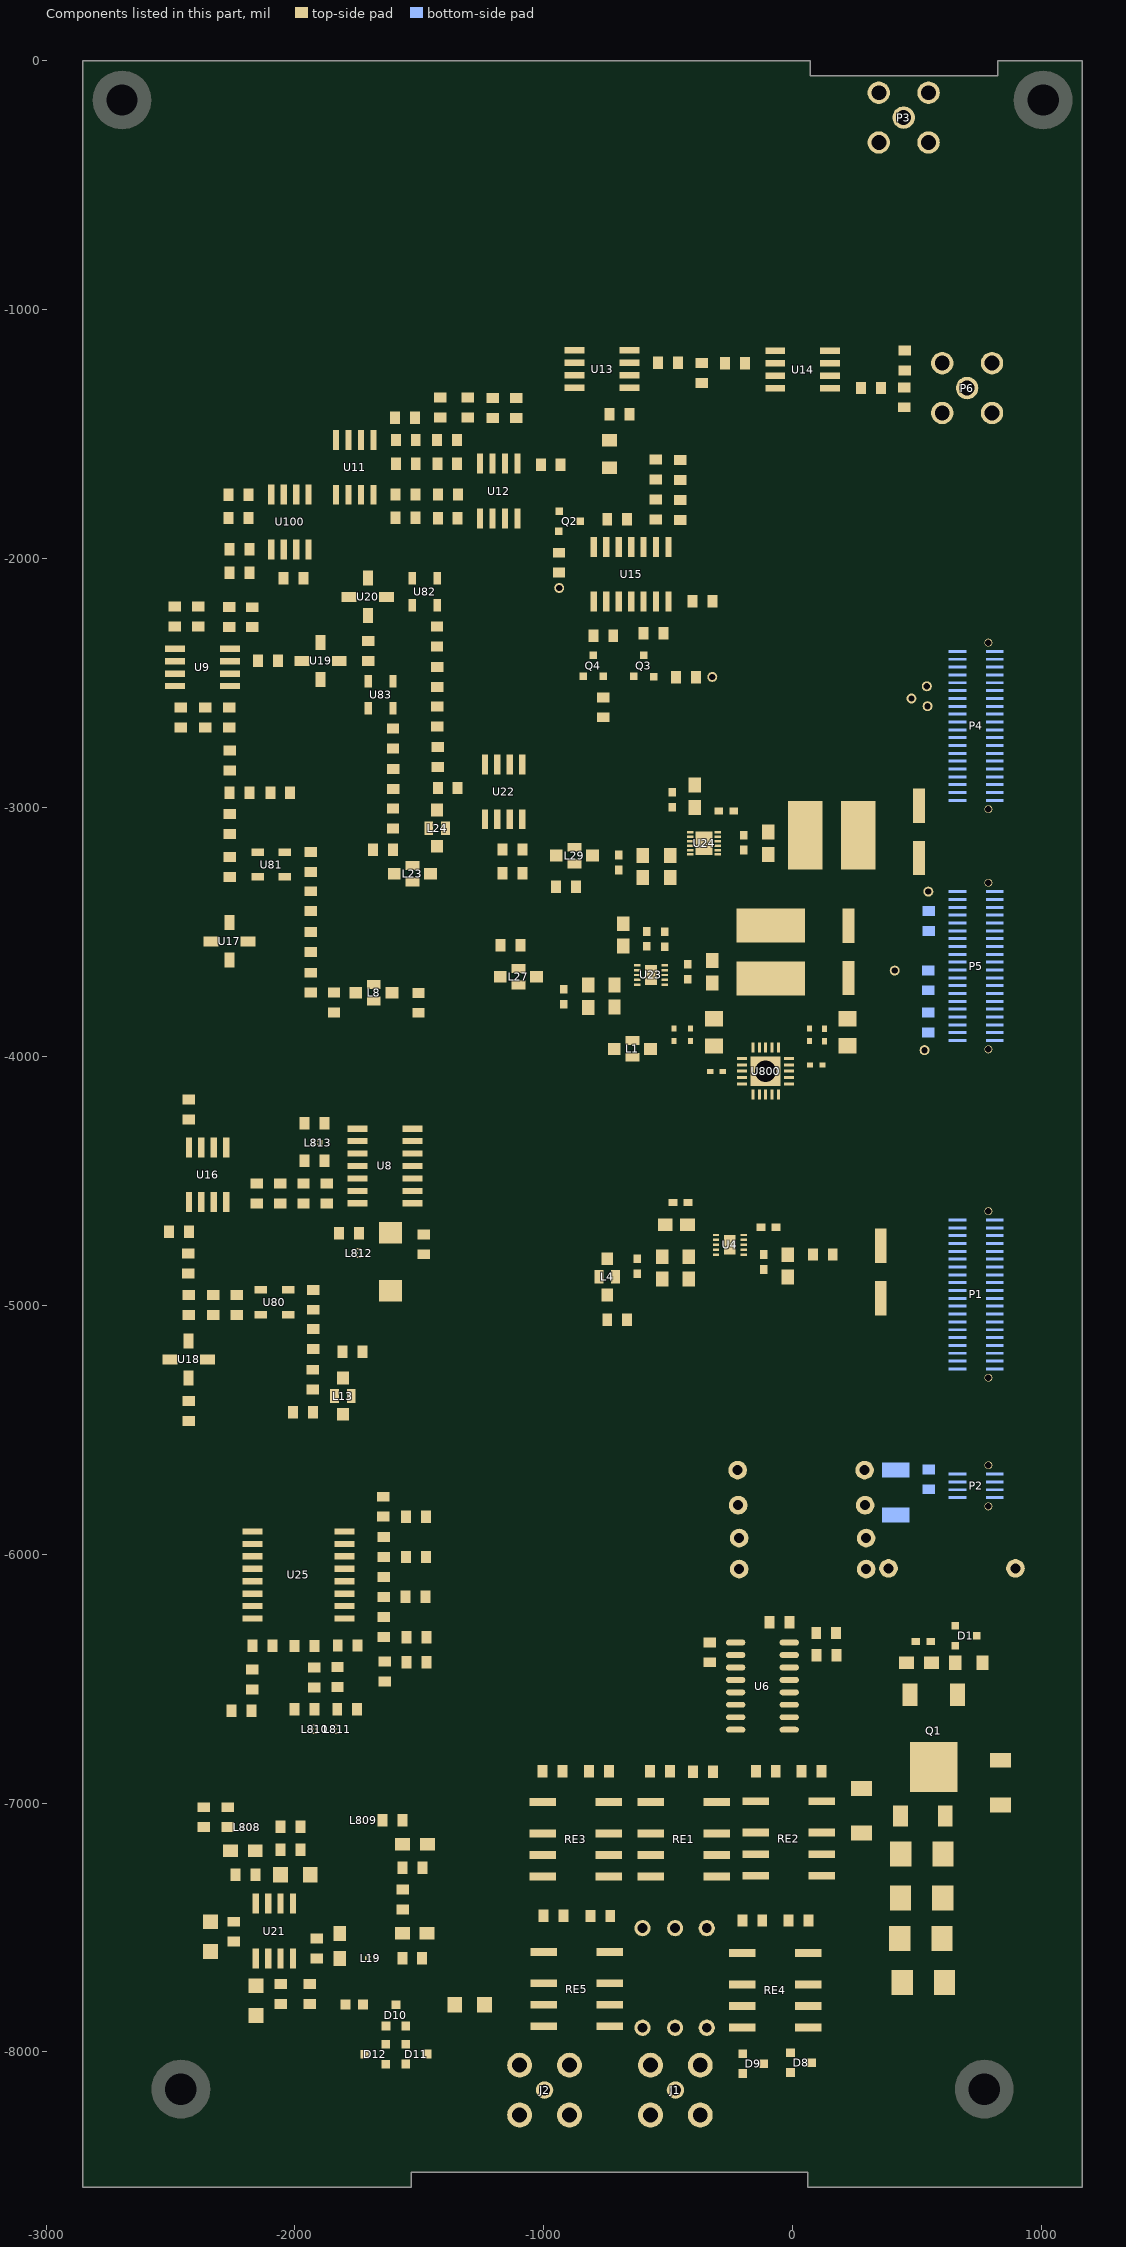
[diagram p0: the components of this part, seen from the top]
# Altium PCB MISC109560.PcbDoc (part 7 of 7)
Units mil, origin at the board's own origin, x right, y up, seen from the top; angles counter-clockwise.
Board outline 4015.75 x 8543.31 mil, 4 copper layers (TopLayer, GND, SIG3, BottomLayer); 280 components, 173 nets, 936 pads, 3695 vias.

## Polygon pours and split planes (outlines as drawn) (continued)
NetC110_2 on TopLayer "Bottom Layer-No Net" (solid, remove dead copper, pour order 1011): -830,-3163 -830,-3217 -826,-3221 -822,-3225 -794,-3225 -746,-3225 -738,-3217 -729,-3208 -702,-3208 -654,-3208 -647,-3215 -640,-3222 -614,-3222 -406,-3222 -402,-3218 -398,-3214 -398,-3178 -398,-3149 -399,-3148 -401,-3148 -823,-3148 -827,-3152 -830,-3155 -830,-3163
+12V on TopLayer "Bottom Layer-No Net" (solid, remove dead copper, pour order 1012): -1636,-3711 -1636,-3766 -1634,-3768 -1631,-3771 -1603,-3771 -1442,-3771 -1427,-3786 -1423,-3790 -1423,-3828 -1423,-3869 -1413,-3879 -1395,-3897 -1352,-3897 -1199,-3897 -1181,-3915 -1173,-3923 -1173,-3968 -1173,-3999 -1166,-4006 -1132,-4040 -904,-4040 -704,-4040 -695,-4031 -690,-4026 -690,-3997 -690,-3938 -691,-3937 -696,-3932 -731,-3932 -1039,-3932 -1050,-3921 -1059,-3912 -1059,-3888 -1059,-3840 -1083,-3816 -1102,-3797 -1170,-3797 -1257,-3797 -1280,-3774 -1293,-3761 -1293,-3714 -1293,-3476 -1293,-3471 -1241,-3419 -1231,-3409 -1160,-3409 -1074,-3409 -1065,-3400 -1048,-3383 -1048,-3268 -1048,-3149 -1055,-3142 -1056,-3141 -1063,-3141 -1102,-3141 -1107,-3146 -1107,-3151 -1107,-3305 -1123,-3321 -1129,-3327 -1175,-3327 -1251,-3327 -1323,-3399 -1370,-3446 -1370,-3530 -1370,-3661 -1381,-3672 -1399,-3690 -1510,-3690 -1624,-3690 -1633,-3699 -1636,-3702 -1636,-3711
+5V on TopLayer "Bottom Layer-No Net" (solid, remove dead copper, pour order 1013): -1255,-3649 -1255,-3699 -1246,-3708 -1240,-3714 -1208,-3714 -1154,-3714 -1148,-3708 -1148,-3674 -1148,-3531 -1151,-3528 -1154,-3525 -1167,-3525 -1197,-3525 -1202,-3530 -1255,-3583 -1255,-3649
-5V on TopLayer "Bottom Layer-No Net" (solid, remove dead copper, pour order 1014): -1017,-3276 -1017,-3349 -1012,-3354 -1007,-3359 -998,-3359 -939,-3359 -934,-3354 -924,-3344 -924,-3217 -924,-3168 -927,-3165 -930,-3162 -939,-3162 -990,-3162 -995,-3167 -1017,-3189 -1017,-3276
GND on BottomLayer "Bottom Layer-No Net" (solid, remove dead copper, pour order 1020): -3191,-3960 -3191,-8552 -3011,-8732 -2847,-8896 -2458,-8896 1357,-8896 1387,-8866 1806,-8447 1806,-8223 1806,-6391 1787,-6372 1649,-6234 789,-6234 -267,-6234 -339,-6162 -362,-6139 -362,-6071 -362,-5565 -265,-5468 -255,-5458 -219,-5458 1268,-5458 1308,-5418 1387,-5339 1387,-5250 1387,214 1372,229 1013,588 -244,588 -2473,588 -2682,379 -3191,-130 -3191,-3960
HT on BottomLayer "Bottom Layer-No Net" (solid, remove dead copper, pour order 1055): 509,-5736.31 509,-5748.31 509,-5799.31 512,-5802.31 528,-5818.31 542,-5818.31 688,-5818.31 696,-5810.31 706,-5800.31 706,-5769.31 706,-5671.31 701,-5666.31 699,-5664.31 622,-5664.31 616,-5670.31 615,-5671.31 615,-5684.31 615,-5691.31 606,-5700.31 594,-5712.31 552,-5712.31 519,-5712.31 515,-5716.31 509,-5722.31 509,-5736.31
+12.5V on BottomLayer "Bottom Layer-No Net" (solid, remove dead copper, pour order 1059): 503,-3913.31 503,-3989.31 507,-3993.31 514,-4000.31 534,-4000.31 566,-4000.31 580,-3986.31 623,-3943.31 686,-3943.31 849,-3943.31 852,-3940.31 859,-3933.31 859,-3915.31 859,-3815.31 851,-3807.31 848,-3804.31 822,-3804.31 613,-3804.31 606,-3811.31 603,-3814.31 603,-3822.31 603,-3863.31 590,-3876.31 584,-3882.31 551,-3882.31 521,-3882.31 508,-3895.31 503,-3900.31 503,-3912.31
A6V on BottomLayer "Bottom Layer-No Net" (solid, remove dead copper, pour order 1057): 369,-3529.31 369,-3665.31 380,-3676.31 545,-3676.31 595,-3676.31 607,-3688.31 610,-3691.31 637,-3691.31 850,-3691.31 854,-3687.31 857,-3684.31 857,-3675.31 857,-3589.31 853,-3585.31 851,-3583.31 846,-3583.31 511,-3583.31 463,-3535.31 445,-3517.31 392,-3517.31 381,-3517.31 369,-3529.31
-5.4V on BottomLayer "Bottom Layer-No Net" (solid, remove dead copper, pour order 1015): 451,-3313 451,-3402 476,-3427 487,-3438 554,-3438 587,-3438 612,-3463 618,-3469 656,-3469 849,-3469 851,-3467 854,-3464 854,-3454 854,-3337 852,-3335 849,-3332 844,-3332 709,-3332 706,-3329 682,-3305 682,-3256 682,-3255 664,-3237 653,-3226 577,-3226 488,-3226 469,-3245 451,-3263 451,-3312
GND on BottomLayer "Bottom Layer-No Net" (solid, remove dead copper, pour order 1016): 361,-5835 361,-5887 367,-5893 402,-5928 522,-5928 873,-5928 886,-5915 928,-5873 928,-5713 928,-5323 923,-5318 918,-5313 908,-5313 864,-5313 861,-5316 853,-5324 853,-5332 853,-5416 859,-5422 867,-5430 867,-5466 867,-5648 853,-5662 844,-5671 801,-5671 769,-5671 762,-5678 759,-5681 759,-5694 759,-5766 769,-5776 771,-5778 785,-5778 808,-5778 818,-5788 820,-5790 820,-5805 820,-5840 811,-5849 800.67,-5859.33 763,-5859.33 522.33,-5859.33 480,-5817 473,-5810 457,-5810 365,-5810 361,-5814 361,-5835
A6V on SIG3 "Bottom Layer-No Net" (solid, remove dead copper, pour order 1017): 366,-3565 366,-3669 378,-3681 386,-3689 430,-3689 590,-3689 617,-3716 630,-3729 630,-3797 630,-4426 559,-4497 527,-4529 291,-4529 180,-4529 155,-4554 148,-4561 148,-4636 148,-4743 173,-4768 188,-4783 312,-4783 869,-4783 880,-4772 923,-4729 923,-4517 923,-3583 878,-3538 811,-3471 612,-3471 409,-3471 380,-3500 366,-3514 366,-3563
+5V on SIG3 "Bottom Layer-No Net" (solid, remove dead copper, pour order 1018): -1263,-3660 -1263,-3697 -1259,-3701 -1252,-3708 -1246,-3708 -1221,-3708 -1215,-3702 -1209,-3696 -1209,-3692 -1209,-3655 -1215,-3649 -1219,-3645 -1228,-3645 -1256,-3645 -1259,-3648 -1263,-3652 -1263,-3659
GND on SIG3 "Bottom Layer-No Net" (solid, remove dead copper, pour order 1019): -3191,-3960 -3191,-8552 -3011,-8732 -2847,-8896 -2458,-8896 1357,-8896 1387,-8866 1806,-8447 1806,-8223 1806,-6391 1787,-6372 1649,-6234 789,-6234 -267,-6234 -339,-6162 -362,-6139 -362,-6071 -362,-5565 -265,-5468 -255,-5458 -219,-5458 1268,-5458 1308,-5418 1387,-5339 1387,-5250 1387,214 1372,229 1013,588 -244,588 -2473,588 -2682,379 -3191,-130 -3191,-3960
GND on GND "Bottom Layer-No Net" (solid, remove dead copper, pour order 1020): -3191,-3960 -3191,-8552 -3011,-8732 -2847,-8896 -2458,-8896 1357,-8896 1387,-8866 1806,-8447 1806,-8223 1806,-6391 1787,-6372 1649,-6234 789,-6234 -267,-6234 -339,-6162 -362,-6139 -362,-6071 -362,-5565 -265,-5468 -255,-5458 -219,-5458 1268,-5458 1308,-5418 1387,-5339 1387,-5250 1387,214 1372,229 1013,588 -244,588 -2473,588 -2682,379 -3191,-130 -3191,-3960

## Keep-outs
KeepOutLayer:
  lines w5: -339,-6127.31 -339,-5578.31 -242,-5481.31 847,-5481.31 847,-5551.31 -210,-5551.31 -274,-5615.31 -274,-6096.31 -234,-6136.31 838,-6136.31 838,-6211.31 -255,-6211.31 -339,-6127.31
  lines w10: -2852,-8543.31 -1532.7,-8543.31 -1532.7,-8484.25 60.7,-8484.25 60.7,-8543.31 1163.75,-8543.31 1163.75,0 824.22,0 824.22,-59.06 70.78,-59.06 70.78,0 -2852,0 -2852,-8543.31

## Other copper
TopLayer:
  rectangle net GND: -2380,-4119.28 -1205,-3923.61
  rectangle net GND: -2713,-4120.85 -2480,-3924
  rectangle net GND: -1402.4,-8365 -1205.16,-7878
  rectangle net GND: -1280,-4439.31 1144,-4245.31
  rectangle net GND: 949,-8471 1144,-4245.31
  rectangle net GND: -2834,-8471.31 1125,-8311
  rectangle net GND: -2836.25,-8470 -2639.4,-393
  rectangle net GND: -1401.61,-7742 -1205.16,-4062
  rectangle net GND: 950.76,-4287 1146.43,-393
  rectangle net GND: -2838.68,-589.85 646,-393.39
  rectangle net GND: 637.57,-589.46 1144,-393
  rectangle net GND: -2808,-5726.85 -2492,-5530
  rectangle net GND: -2356,-5725.28 -1377.29,-5529.61
  rectangle net GND: -2735.44,-6947.61 -2109,-6751.15
  rectangle net GND: -2013,-6948.39 -1362.21,-6752.33
BottomLayer:
  rectangle net GND: -2380,-4119.28 -1205,-3923.61
  rectangle net GND: -2712,-4120.85 -1207,-3924
  rectangle net GND: -1280,-4439.31 1144,-4245.31
  rectangle net GND: 949,-8472 1144,-4245.31
  rectangle net GND: -2834,-8471.31 1125,-8311
  rectangle net GND: -2836.25,-8466 -2639.4,-393
  rectangle net GND: -1401.61,-8358 -1205.16,-4062
  rectangle net GND: 950.76,-4258 1146.43,-393
  rectangle net GND: -2838.68,-589.85 647,-393.39
  rectangle net GND: 637.57,-589.46 1144,-393
  rectangle net GND: -2808,-5725 -2349,-5530
  rectangle net GND: -2356,-5725.28 -1377.29,-5529.61
  rectangle net GND: -2735.44,-6947.61 -2004,-6751.15
  rectangle net GND: -2013,-6948.39 -1362.21,-6752.33

## Silkscreen, mask and mechanical layers (free items; w line width, h text height)
TopSolder:
  rectangle: -2806.56,-4120.85 -2479,-3924
  rectangle: -2380,-4118.67 -1216,-3923
  rectangle: -1401.24,-8467.09 -1204,-7878
  rectangle: -2693,-8471.31 1144,-8311
  rectangle: 949,-8401 1144,-4245.31
  rectangle: -2836.25,-8470 -2639.4,-393
  rectangle: -1401.46,-7741 -1205,-3923
  rectangle: -1387,-4439 1146.04,-4242.94
  rectangle: 950.76,-4281 1146.43,-393
  rectangle: -2838.68,-589.85 653,-393.39
  rectangle: 637.57,-589.46 1144,-393
  rectangle: -2819.56,-5726.85 -2492,-5530
  rectangle: -2356,-5724.67 -1402.46,-5529
  rectangle: -2727,-6947 -2109,-6750.54
  rectangle: -2013,-6949.06 -1274,-6753
BottomSolder:
  rectangle: -2807.56,-4120.85 -2373,-3924
  rectangle: -2379,-4121 -1206,-3924
  rectangle: -2836,-8471.31 1125,-8311
  rectangle: 949,-8472 1144,-4245.31
  rectangle: -2836.25,-8361 -2639.4,-393
  rectangle: -1402,-8358 -1205.54,-3925
  rectangle: -1392,-4441.06 1148,-4245
  rectangle: 950.76,-4259 1146,-393
  rectangle: -2838.68,-589.85 798,-393.39
  rectangle: 638.57,-589.46 1144,-393
  rectangle: -2819.56,-5727 -2333,-5530.15
  rectangle: -2356,-5726 -1388,-5529
  rectangle: -2655,-6948 -1987,-6751.54
  rectangle: -2013,-6948.06 -1227.57,-6752